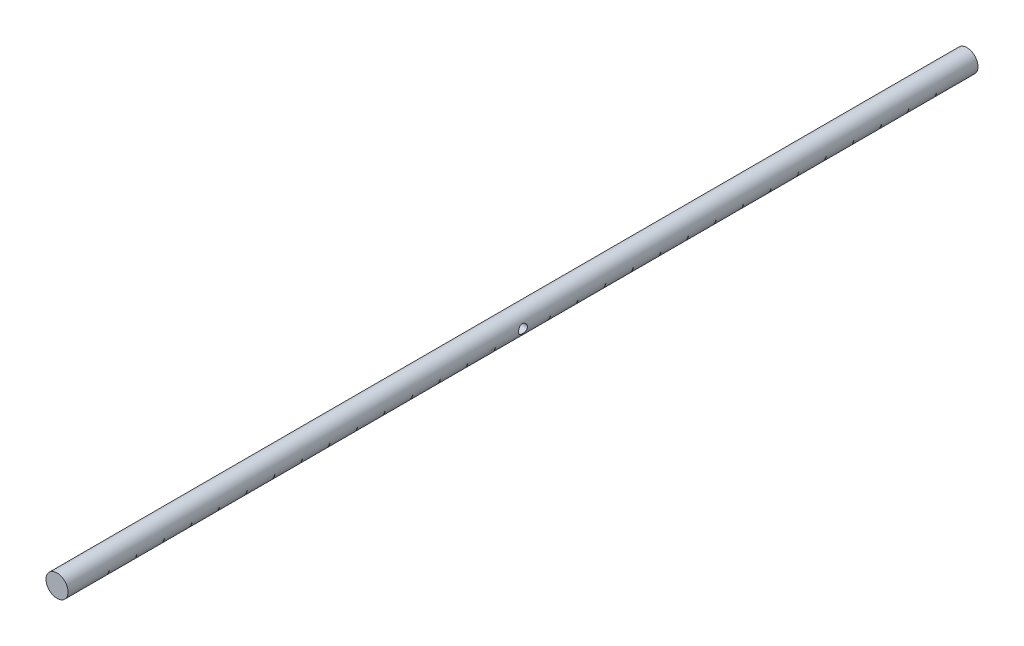
from build123d import *

# Parameters (mm, degrees)
SKETCH1_R           = 4
BOSS_EXTRUDE1_DEPTH = 330
SKETCH2_R           = 1.6
CUT_EXTRUDE1_DEPTH  = 331.121189868
CUT_EXTRUDE2_DEPTH  = 0.1
LPATTERN1_COUNT     = 31
LPATTERN1_PITCH     = 5
LPATTERN1_COL_COUNT = 31
LPATTERN1_COL_PITCH = 5
CUT_EXTRUDE3_DEPTH  = 0.1
LPATTERN2_COUNT     = 16
LPATTERN2_PITCH     = 10
LPATTERN2_COL_COUNT = 16
LPATTERN2_COL_PITCH = 10


with BuildPart() as part:
    # Sketch1 → Boss-Extrude1 (new body)
    with BuildSketch(Plane.XY):
        Circle(SKETCH1_R)
    extrude(amount=BOSS_EXTRUDE1_DEPTH)

    # Sketch2 → Cut-Extrude1 (cut, through all)
    with BuildSketch(Plane(origin=(4, 0, 0), x_dir=(0, 0, -1), z_dir=(1, 0, 0))):
        with Locations((-165, 0)):
            Circle(SKETCH2_R)
    extrude(amount=-CUT_EXTRUDE1_DEPTH, mode=Mode.SUBTRACT)

    # Sketch6 → Cut-Extrude2 (cut, symmetric)
    with BuildSketch(Plane(origin=(0, 0, 165), x_dir=(-1, 0, 0), z_dir=(0, 0, -1))):
        with BuildLine():
            Line((-2.987573328, -2.506871678), (-3.447199994, -2.892544244))
            ThreePointArc((-3.447199994, -2.892544244), (-1.901782178, -4.078385042), (0, -4.5))
            Line((0, -4.5), (0, -3.9))
            ThreePointArc((0, -3.9), (-1.648211221, -3.534600369), (-2.987573328, -2.506871678))
        make_face()
    cut_extrude2 = extrude(amount=CUT_EXTRUDE2_DEPTH, both=True, mode=Mode.SUBTRACT)

    # LPattern1: Cut-Extrude2 ×31
    with Locations(*[(0, 0, -i * LPATTERN1_PITCH) for i in range(1, LPATTERN1_COUNT)]):
        add(cut_extrude2, mode=Mode.SUBTRACT)

    # LPattern1 col: Cut-Extrude2 ×31
    with Locations(*[(0, 0, i * LPATTERN1_COL_PITCH) for i in range(1, LPATTERN1_COL_COUNT)]):
        add(cut_extrude2, mode=Mode.SUBTRACT)

    # Sketch7 → Cut-Extrude3 (cut, symmetric)
    with BuildSketch(Plane.XY.offset(165)):
        with BuildLine():
            Line((3.840750237, -0.677227893), (4.431634889, -0.7814168))
            ThreePointArc((4.431634889, -0.7814168), (2.892544244, -3.447199994), (0, -4.5))
            Line((0, -4.5), (0, -3.9))
            ThreePointArc((0, -3.9), (2.506871678, -2.987573328), (3.840750237, -0.677227893))
        make_face()
    cut_extrude3 = extrude(amount=CUT_EXTRUDE3_DEPTH, both=True, mode=Mode.SUBTRACT)

    # LPattern2: Cut-Extrude3 ×16
    with Locations(*[(0, 0, i * LPATTERN2_PITCH) for i in range(1, LPATTERN2_COUNT)]):
        add(cut_extrude3, mode=Mode.SUBTRACT)

    # LPattern2 col: Cut-Extrude3 ×16
    with Locations(*[(0, 0, -i * LPATTERN2_COL_PITCH) for i in range(1, LPATTERN2_COL_COUNT)]):
        add(cut_extrude3, mode=Mode.SUBTRACT)


solid = part.part
